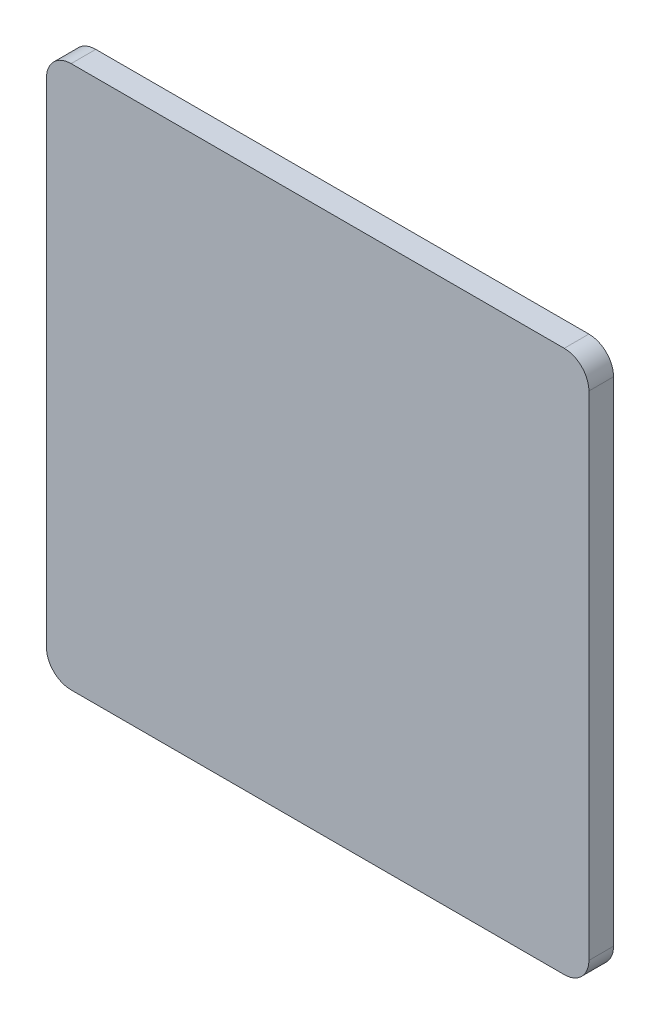
from build123d import *

# Parameters (mm, degrees)
SKETCH_1_W      = 220
SKETCH_1_H      = 220
EXTRUDE_1_DEPTH = 10
FILLET_1_R      = 10


with BuildPart() as part:
    # 草图1 → 凸台-拉伸1 (new body)
    with BuildSketch(Plane.XY):
        Rectangle(SKETCH_1_W, SKETCH_1_H)
    extrude(amount=EXTRUDE_1_DEPTH)

    # 圆角1
    fillet_1_edges = [part.edges().sort_by_distance(p)[0] for p in [
        (-110, 110, 5),
        (110, 110, 5),
        (110, -110, 5),
        (-110, -110, 5),
    ]]
    fillet(fillet_1_edges, radius=FILLET_1_R)


solid = part.part
